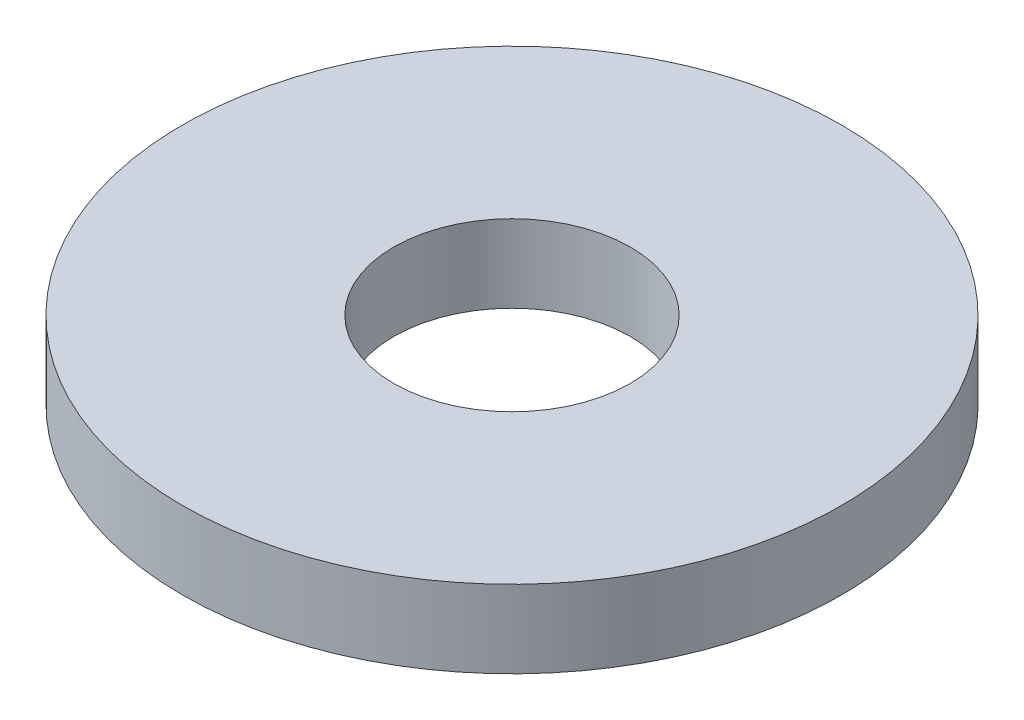
from build123d import *

# Parameters (mm, degrees)
SKETCH1_R           = 4.25
SKETCH1_R_2         = 1.525
BOSS_EXTRUDE1_DEPTH = 1


with BuildPart() as part:
    # Sketch1 → Boss-Extrude1 (new body)
    with BuildSketch(Plane(origin=(0, 0, 0), x_dir=(1, 0, 0), z_dir=(0, 1, 0))):
        with Locations(Location((0, 0, 0), (0, 0, 270))):
            Circle(SKETCH1_R)
        with Locations(Location((0, 0, 0), (0, 0, 270))):
            Circle(SKETCH1_R_2, mode=Mode.SUBTRACT)
    extrude(amount=BOSS_EXTRUDE1_DEPTH)


solid = part.part
